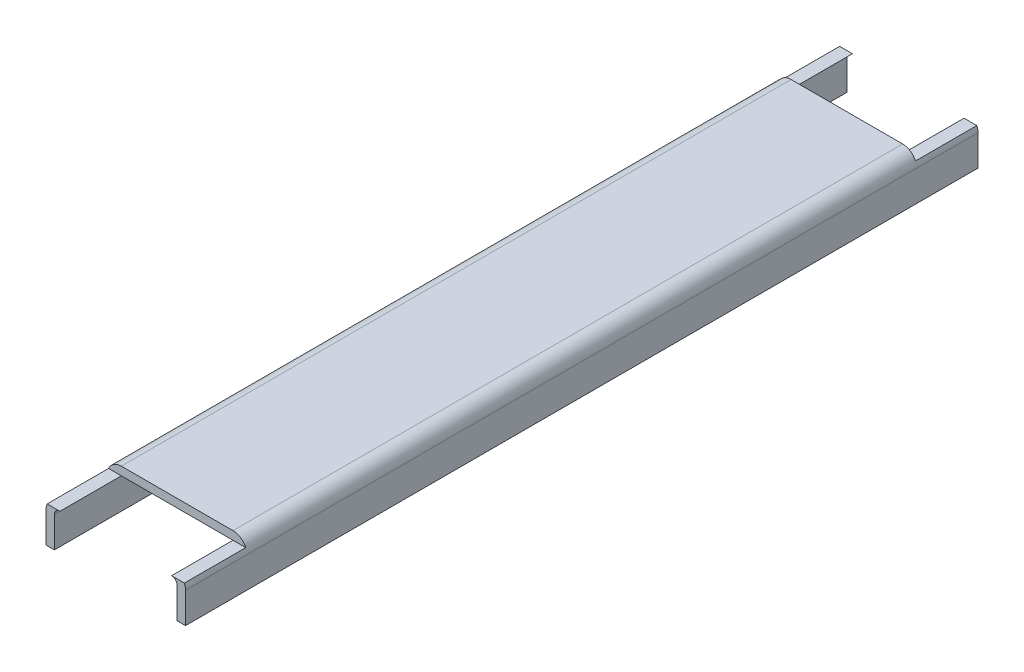
from build123d import *

# Parameters (mm, degrees)
BOSS_EXTRUDE1_DEPTH = 568
CUT_EXTRUDE1_DEPTH  = 44
CUT_EXTRUDE2_DEPTH  = 44


with BuildPart() as part:
    # Sketch1 → Boss-Extrude1 (new body)
    with BuildSketch(Plane.XY):
        with BuildLine():
            Line((0, 0), (0, 22))
            ThreePointArc((0, 22), (2.928932188, 29.071067812), (10, 32))
            Line((10, 32), (90, 32))
            ThreePointArc((90, 32), (97.071067812, 29.071067812), (100, 22))
            Line((100, 22), (100, 0))
            Line((100, 0), (94, 0))
            Line((94, 0), (94, 22))
            ThreePointArc((94, 22), (92.828427125, 24.828427125), (90, 26))
            Line((90, 26), (10, 26))
            ThreePointArc((10, 26), (7.171572875, 24.828427125), (6, 22))
            Line((6, 22), (6, 0))
            Line((6, 0), (0, 0))
        make_face()
    extrude(amount=BOSS_EXTRUDE1_DEPTH)

    # Sketch2 → Cut-Extrude1 (cut)
    with BuildSketch(Plane.XY.offset(568)):
        Polygon((-5.016704774, 26), (110.589606684, 26), (113.542758838, 46.117705453), (4.096772107, 46.117705453), (-12.020365044, 28.61582492), align=None)
    extrude(amount=-CUT_EXTRUDE1_DEPTH, mode=Mode.SUBTRACT)

    # Sketch3 → Cut-Extrude2 (cut)
    with BuildSketch(Plane(origin=(0, 0, 0), x_dir=(-1, 0, 0), z_dir=(0, 0, -1))):
        Polygon((-112.020365044, 26), (27.466483662, 26), (17.252014884, 45.492114728), (-47.890463774, 56.039795858), (-51.518866083, 56.039795858), (-99.243616331, 54.20535901), align=None)
    extrude(amount=-CUT_EXTRUDE2_DEPTH, mode=Mode.SUBTRACT)


solid = part.part
